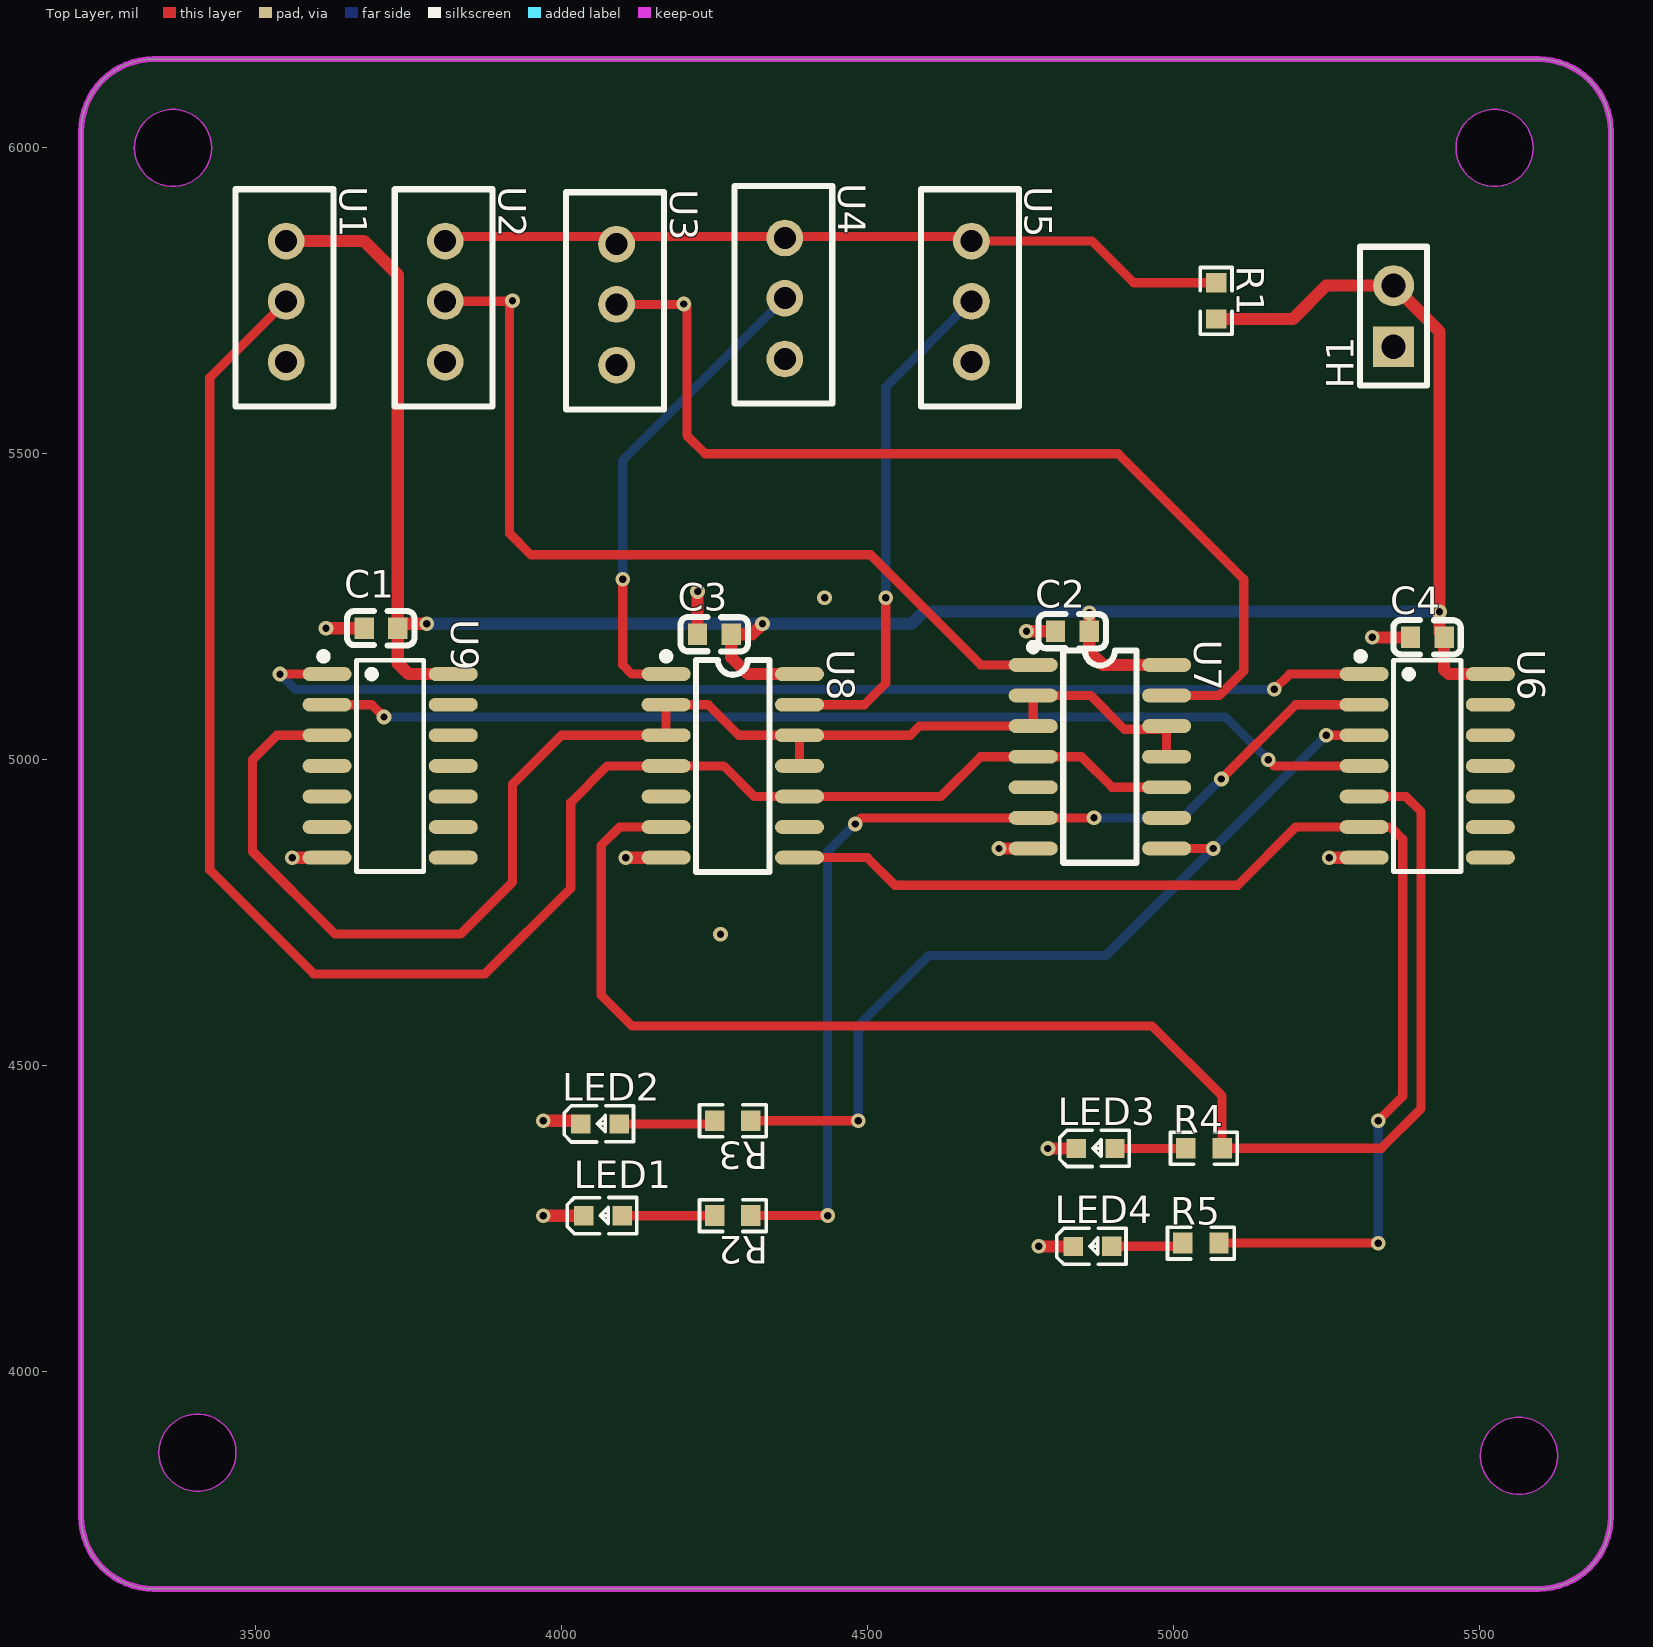
[diagram p0: Top Layer view]
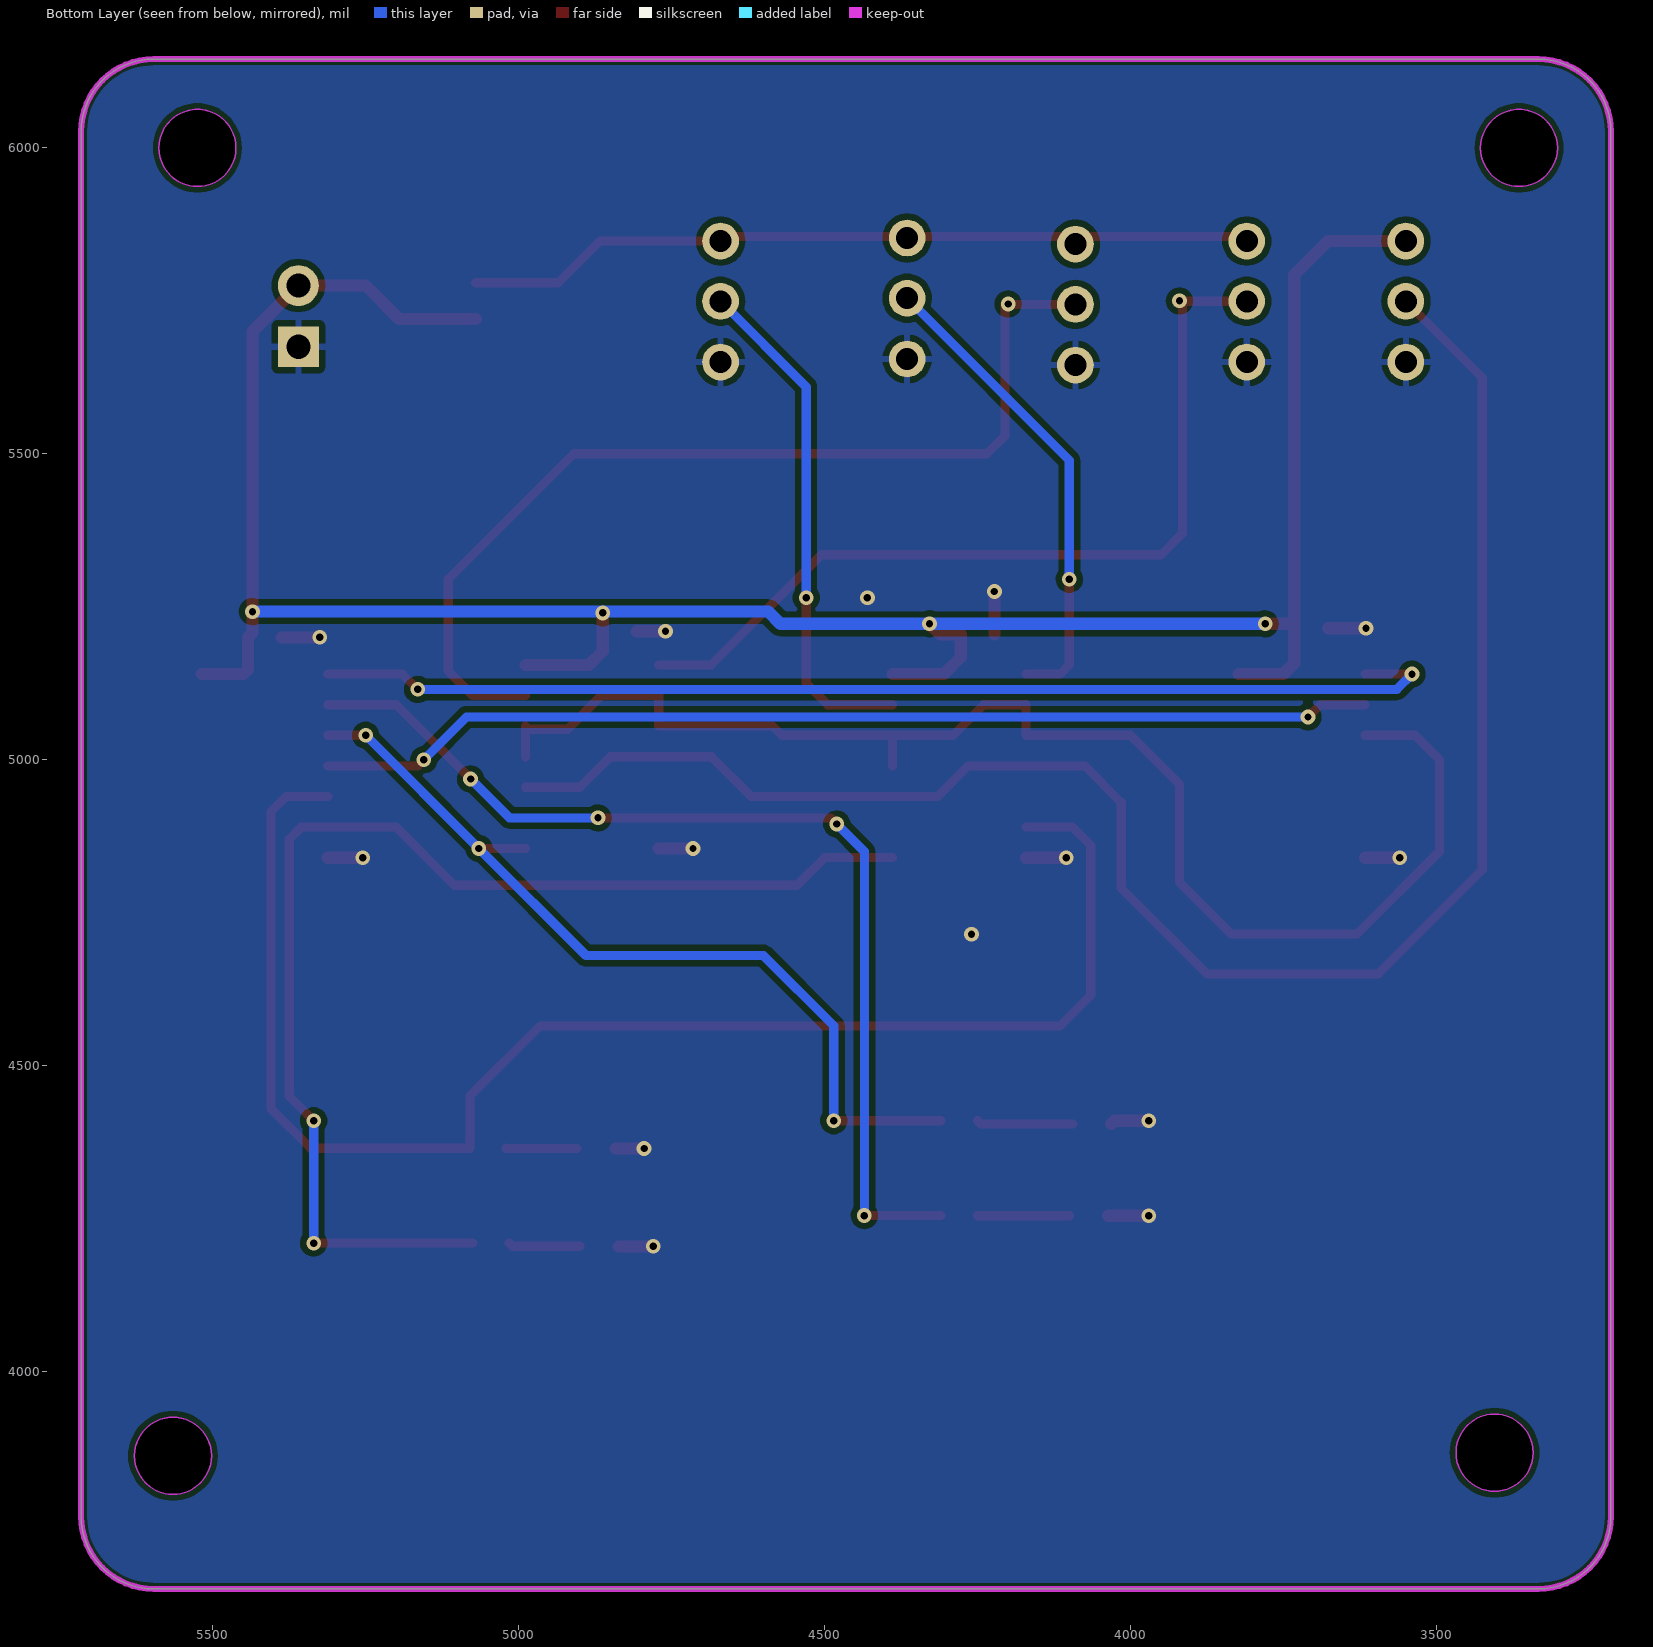
[diagram p1: Bottom Layer view, seen from below]
# Altium PCB MISC51255.pcbdoc
Units mil, origin at the board's own origin, x right, y up, seen from the top; angles counter-clockwise.
Board outline 2500 x 2500 mil, 2 copper layers (Top Layer, Bottom Layer), stack 62.206 mil thick; 23 components, 19 nets, 99 pads, 35 vias.

## Layer stack, top to bottom
Top Solder Mask Layer: solder mask 0.394, Dk 3.3
Top Layer: signal copper 1.379
Dielectric1: surface 59.449, FR4, Dk 4.5
Bottom Layer: signal copper 1.378
Bottom Solder Mask Layer: solder mask 0.394, Dk 3.3

## Board outline
3333.1,6145 ccw(c3333.1,6026.9) 3215,6026.9 3215,3763.1 ccw(c3333.1,3763.1) 3333.1,3645 5596.9,3645 ccw(c5596.9,3763.1) 5715,3763.1 5715,6026.9 ccw(c5596.9,6026.9) 5596.9,6145 3333.1,6145
cut-out: 3428,6000 cw(c3365,6000) 3302,6000 cw(c3365,6000)
cut-out: 5588,6000 cw(c5525,6000) 5462,6000 cw(c5525,6000)
cut-out: 3468,3867.44 cw(c3405,3867.44) 3342,3867.44 cw(c3405,3867.44)
cut-out: 5628,3862.44 cw(c5565,3862.44) 5502,3862.44 cw(c5565,3862.44)

## Design rules (kind name [scope] priority, off if disabled: settings)
BoardOutlineClearance copperThickness2oz_1 [All] p2 off: genericclearance=7.99 ignorepadtopadclearanceinfootprint=FALSE except(0: Arc-SplitContinuation Track-SplitContinuation SMDPad-SplitContinuation THPad-SplitContinuation Via-SplitContinuation Fill-SplitContinuation Region-SplitContinuation Poly-SplitContinuation Text-SplitContinuation Hole-SplitContinuation; 5.98: Arc-CutoutEdge SMDPad-CutoutEdge THPad-CutoutEdge Via-CutoutEdge Fill-CutoutEdge Region-CutoutEdge Text-CutoutEdge; 6.93: Hole-OutlineEdge Hole-CutoutEdge; 10: Poly-OutlineEdge Poly-CutoutEdge; 11.81: Arc-OutlineEdge Track-OutlineEdge SMDPad-OutlineEdge THPad-OutlineEdge Via-OutlineEdge Fill-OutlineEdge Region-OutlineEdge Text-OutlineEdge Track-CutoutEdge)
BoardOutlineClearance Plane_innerPlane_1 [All] p4 off: genericclearance=4.02 ignorepadtopadclearanceinfootprint=FALSE except(0: Arc-SplitContinuation Track-SplitContinuation SMDPad-SplitContinuation THPad-SplitContinuation Via-SplitContinuation Fill-SplitContinuation Region-SplitContinuation Poly-SplitContinuation Text-SplitContinuation Hole-SplitContinuation; 6: SMDPad-CutoutEdge THPad-CutoutEdge Via-CutoutEdge Fill-CutoutEdge Region-CutoutEdge Text-CutoutEdge; 6.93: Hole-OutlineEdge Hole-CutoutEdge; 10: Poly-OutlineEdge Poly-CutoutEdge; 11.8: Arc-OutlineEdge Track-OutlineEdge SMDPad-OutlineEdge THPad-OutlineEdge Via-OutlineEdge Fill-OutlineEdge Region-OutlineEdge Text-OutlineEdge; 11.81: Arc-CutoutEdge Track-CutoutEdge)
BoardOutlineClearance Copper_copperRegion_1 [All] p6 off: genericclearance=4.02 ignorepadtopadclearanceinfootprint=FALSE except(0: Arc-SplitContinuation Track-SplitContinuation SMDPad-SplitContinuation THPad-SplitContinuation Via-SplitContinuation Fill-SplitContinuation Region-SplitContinuation Poly-SplitContinuation Text-SplitContinuation Hole-SplitContinuation; 6: SMDPad-CutoutEdge THPad-CutoutEdge Via-CutoutEdge Fill-CutoutEdge Region-CutoutEdge Text-CutoutEdge; 6.93: Hole-OutlineEdge Hole-CutoutEdge; 10: Poly-OutlineEdge Poly-CutoutEdge; 11.8: Arc-OutlineEdge Track-OutlineEdge SMDPad-OutlineEdge THPad-OutlineEdge Via-OutlineEdge Fill-OutlineEdge Region-OutlineEdge Text-OutlineEdge; 11.81: Arc-CutoutEdge Track-CutoutEdge)
BoardOutlineClearance copperThickness1oz_1 [All] p8: genericclearance=4.02 ignorepadtopadclearanceinfootprint=FALSE except(0: Arc-SplitContinuation Track-SplitContinuation SMDPad-SplitContinuation THPad-SplitContinuation Via-SplitContinuation Fill-SplitContinuation Region-SplitContinuation Poly-SplitContinuation Text-SplitContinuation Hole-SplitContinuation; 6: SMDPad-CutoutEdge THPad-CutoutEdge Via-CutoutEdge Fill-CutoutEdge Region-CutoutEdge Text-CutoutEdge; 6.93: Hole-OutlineEdge Hole-CutoutEdge; 10: Poly-OutlineEdge Poly-CutoutEdge; 11.8: Arc-OutlineEdge Track-OutlineEdge SMDPad-OutlineEdge THPad-OutlineEdge Via-OutlineEdge Fill-OutlineEdge Region-OutlineEdge Text-OutlineEdge; 11.81: Arc-CutoutEdge Track-CutoutEdge)
Clearance copperThickness2oz [All] p1 off: gap=7.99 ignorepadtopadclearanceinfootprint=FALSE except(5.98: SMDPad-Track SMDPad-SMDPad THPad-Track SMDPad-THPad THPad-THPad Track-Via SMDPad-Via THPad-Via Via-Via Fill-Track Region-Track Fill-SMDPad Region-SMDPad Fill-THPad Region-THPad Fill-Via Region-Via Fill-Fill Fill-Region Region-Region Arc-Track Arc-SMDPad Arc-THPad Arc-Via Fill-Arc Region-Arc Arc-Arc Text-Track SMDPad-Text Text-THPad Text-Via Fill-Text Region-Text Arc-Text Text-Text; 6.93: Hole-Track Hole-SMDPad Hole-THPad Hole-Via Fill-Hole Region-Hole Hole-Arc Hole-Text; 10: Poly-Track Poly-SMDPad Poly-THPad Poly-Via Poly-Fill Poly-Region Poly-Poly Poly-Arc Poly-Text Poly-Hole)
Clearance Plane_innerPlane [All] p3 off: gap=4.02 ignorepadtopadclearanceinfootprint=FALSE except(5.98: SMDPad-Track SMDPad-SMDPad THPad-Track SMDPad-THPad THPad-THPad Track-Via SMDPad-Via THPad-Via Via-Via Fill-Track Region-Track Fill-SMDPad Region-SMDPad Fill-THPad Region-THPad Fill-Via Region-Via Fill-Fill Fill-Region Region-Region; 6: Arc-Track Arc-SMDPad Arc-THPad Arc-Via Fill-Arc Region-Arc Arc-Arc Text-Track SMDPad-Text Text-THPad Text-Via Fill-Text Region-Text Arc-Text Text-Text; 6.93: Hole-Track Hole-SMDPad Hole-THPad Hole-Via Fill-Hole Region-Hole Hole-Arc Hole-Text; 10: Poly-Track Poly-SMDPad Poly-THPad Poly-Via Poly-Fill Poly-Region Poly-Poly Poly-Arc Poly-Text Poly-Hole)
Clearance Copper_copperRegion [All] p5 off: gap=4.02 ignorepadtopadclearanceinfootprint=FALSE except(5.98: SMDPad-Track SMDPad-SMDPad THPad-Track SMDPad-THPad THPad-THPad Track-Via SMDPad-Via THPad-Via Via-Via Fill-Track Region-Track Fill-SMDPad Region-SMDPad Fill-THPad Region-THPad Fill-Via Region-Via Fill-Fill Fill-Region Region-Region; 6: Arc-Track Arc-SMDPad Arc-THPad Arc-Via Fill-Arc Region-Arc Arc-Arc Text-Track SMDPad-Text Text-THPad Text-Via Fill-Text Region-Text Arc-Text Text-Text; 6.93: Hole-Track Hole-SMDPad Hole-THPad Hole-Via Fill-Hole Region-Hole Hole-Arc Hole-Text; 10: Poly-Track Poly-SMDPad Poly-THPad Poly-Via Poly-Fill Poly-Region Poly-Poly Poly-Arc Poly-Text Poly-Hole)
Clearance copperThickness1oz [All] p7: gap=4.02 ignorepadtopadclearanceinfootprint=FALSE except(5.98: SMDPad-Track SMDPad-SMDPad THPad-Track SMDPad-THPad THPad-THPad Track-Via SMDPad-Via THPad-Via Via-Via Fill-Track Region-Track Fill-SMDPad Region-SMDPad Fill-THPad Region-THPad Fill-Via Region-Via Fill-Fill Fill-Region Region-Region; 6: Arc-Track Arc-SMDPad Arc-THPad Arc-Via Fill-Arc Region-Arc Arc-Arc Text-Track SMDPad-Text Text-THPad Text-Via Fill-Text Region-Text Arc-Text Text-Text; 6.93: Hole-Track Hole-SMDPad Hole-THPad Hole-Via Fill-Hole Region-Hole Hole-Arc Hole-Text; 10: Poly-Track Poly-SMDPad Poly-THPad Poly-Via Poly-Fill Poly-Region Poly-Poly Poly-Arc Poly-Text Poly-Hole)
DiffPairsRouting differentialPair [All] p1: maxlimit=6 minlimit=6 mostfreqgap=6 toplayer_minwidth=5 toplayer_prefwidth=10 toplayer_maxwidth=100 toplayer_mingap=6 toplayer_prefgap=6 toplayer_maxgap=6 bottomlayer_minwidth=5 bottomlayer_prefwidth=10 bottomlayer_maxwidth=100 bottomlayer_mingap=6 bottomlayer_prefgap=6 bottomlayer_maxgap=6 maxuncoupledlength=10
HoleToHoleClearance otherClearance [All] p1: gap=11.81 allowstackedmicrovias=TRUE
Length netLength [All] p1: minlimit=0 maxlimit=0
PasteMaskExpansion pasteMaskExpansion [All] p1: expansion=0
PlaneConnect innerPlane [All] p1: planeconnectstyle=Relief reliefexpansion=20 reliefentries=4 reliefconductorwidth=10 reliefairgap=10
PolygonConnect copperRegion [All] p1: connectstyle=Relief reliefconductorwidth=10 reliefentries=4 polygonreliefangle="90 Angle" airgapwidth=10 via.connectstyle=Relief via.reliefconductorwidth=10 via.reliefentries=4 via.polygonreliefangle="90 Angle" via.airgapwidth=10
RoutingVias viaSize [All] p1: holewidth=12.01 width=24.02 viastyle="Through Hole" minholewidth=11.81 minwidth=19.68 maxholewidth=248.03 maxwidth=393.7
SolderMaskExpansion solderMaskExpansion [IsVia] p1: expansion=-1000 istentingtop=TRUE
SolderMaskExpansion solderMaskExpansion [All] p2: expansion=2 istentingtop=FALSE
Width copperThickness2oz_2 [All] p1 off: maxlimit=100 minlimit=8 preferedwidth=10
Width pwr [(InNet('GND') OR InNet('VCC'))] p2: maxlimit=100 minlimit=5 preferedwidth=20
Width copperThickness1oz_2 [All] p3: maxlimit=100 minlimit=5 preferedwidth=15

## Components (designator, comment, footprint, x,y, rotation, side; value= is the part's Value field where it differs from the comment)
C1 "100nF" C0603 3705,5215 r0 top
C2 "100nF" C0603 4835,5210 r0 top
C3 "100nF" C0603 4250,5205 r0 top
C4 "100nF" C0603 5415,5200 r0 top
H1 "" HDR-TH_2P-P2.54-V-F 5360,5725 r90 top
LED1 "" LED_0603 4070,4255 r0 top
LED2 "" LED_0603 4065,4405 r0 top
LED3 "" LED_0603 4875,4365 r0 top
LED4 "" LED_0603 4870,4205 r0 top
R1 "0.1k" R0603 5070,5750 r270 top
R2 "10K" R0603 4280,4255 r180 top
R3 "10K" R0603 4280,4410 r180 top
R4 "10K" R0603 5050,4365 r180 top
R5 "10K" R0603 5045,4210 r180 top
U1 "" 单刀双掷 3680,5995 r270 top
U2 "" 单刀双掷 3940,5995 r270 top
U3 "" 单刀双掷 4220,5990 r270 top
U4 "" 单刀双掷 4495,6000 r270 top
U5 "" 单刀双掷 4800,5995 r270 top
U6 "SN74LS02DRE4" SOIC-14_L8.7-W3.9-P1.27-LS6.0-BL 5415,4990 r270 top
U7 "SN74LS113ADR" SOIC-14_L8.6-W3.9-P1.27-LS6.0-BL 4880,5005 r270 top
U8 "SN74LS113ADR" SOIC-14_L8.6-W3.9-P1.27-LS6.0-BL 4280,4990 r270 top
U9 "SN74LS08DTR(XBLW)" SOIC-14_L8.7-W3.9-P1.27-LS6.0-BL 3720,4990 r270 top

## Footprints (in the part's own frame and the unit in brackets; to place one, negate y for a bottom-side part, rotate by r counter-clockwise, add the part's x,y. Pads: shape width x height; smd on the part's side, far side on the other; paste and mask are expansions set on the pad)
C0603 [mm]
  rect 0.8x0.9 smd: 1(-0.7,0) 2(0.7,0)
  silkscreen extent -1.41,-0.71 1.39,0.72
HDR-TH_2P-P2.54-V-F [mm]
  rect 1.7x1.7 hole 1: 1(-1.27,0)
  round 1.7 hole 1: 2(1.27,0)
  silkscreen extent -2.88,-1.39 2.88,1.4
LED_0603 [mil]
  rect 31.5x31.5 smd paste+0 mask+2: 1(-33.5,-0.4) 2(29.5,-0.2)
  silkscreen extent -61,-30 53,30
R0603 [mil]
  rect 31.75x34.02 smd paste-3937.01 mask+2: 1(-29.66,0) 2(29.66,0)
  silkscreen extent -55,-26 55,26
SOIC-14_L8.6-W3.9-P1.27-LS6.0-BL [mil]
  oval 22.6x80.24 smd: 1(-150,-109.02) 2(-100,-109.02) 3(-50,-109.02) 4(0,-109.02) 5(50,-109.02) 6(100,-109.02) 7(150,-109.02) 8(150,109.02) 9(100,109.02) 10(50,109.02) 11(0,109.02) 12(-50,109.02) 13(-100,109.02) 14(-150,109.02)
  silkscreen extent -185,-115 173,60
SOIC-14_L8.7-W3.9-P1.27-LS6.0-BL [mil]
  oval 22.6x80.24 smd: 1(-150,-103.11) 2(-100,-103.11) 3(-50,-103.11) 4(0,-103.11) 5(50,-103.11) 6(100,-103.11) 7(150,-103.11) 8(150,103.11) 9(100,103.11) 10(50,103.11) 11(0,103.11) 12(-50,103.11) 13(-100,103.11) 14(-150,103.11)
  silkscreen extent -185,-115 172,55
单刀双掷 [mil]
  round 60 hole 36: 1(147.28,-130) 2(245.7,-130) 3(345,-130)
  silkscreen extent 63,-212 418,-52

## Via types
v1: diameter 24.02, hole 12, Top Layer to Bottom Layer, 35 vias

## Nets (pads, with @x,y where several pads share a name; then routed paths per layer and width w, separated by ;. In a path a pad name is that pad's centre, name@x,y a point inside that pad or via, vN(x,y) a via of type N, cw(c..) or ccw(c..) an arc to the next point about the centre after c; other vN are vias at no path point)
$1N6: R1.1 U2.1 U3.1 U4.1 U5.1 | length 1291.2
  Top Layer w15: U2.1 3817.28,5855 U5.1@4670,5855 ; U5.1 4867.28,5847.72 4935.34,5779.66 R1.1
$1N11: LED1.2 R2.2 | length 150.9
  Top Layer w15: LED1.2 4250.14,4254.8 R2.2
$1N12: LED2.2 R3.2 | length 158
  Top Layer w15: LED2.2 4245.14,4404.8 R3.2
$1N13: LED3.2 R4.2 | length 115.9
  Top Layer w15: LED3.2 5020.14,4364.8 R4.2
$1N14: LED4.2 R5.2 | length 118
  Top Layer w15: LED4.2 5010.14,4204.8 R5.2
$1N18: U2.2 U7.1 | length 1436.4
  Top Layer w15: U2.2 v1@3919.3,5749.3 ; v1(3920,5750) v1@3919.3,5749.3 ; U7.1 4685,5155 4505,5335 3950,5335 3915,5370 3915,5745 v1@3919.3,5749.3
$1N19: U3.2 U7.13 | length 1625.2
  Top Layer w15: U3.2 4199.3,5744.3 v1(4200,5745) ; v1@4205,5745 4205,5530 4235,5500 4910,5500 5115,5295 5115,5145 5075,5105 U7.13
$1N21: U4.2 U8.1 | length 786.3
  Top Layer w15: v1(4100,5295) 4100,5155 4115,5140 U8.1
  Bottom Layer w15: v1(4100,5295) 4100,5489.3 U4.2
$1N22: U5.2 U8.13 | length 837.8
  Top Layer w15: U8.13 4495,5090 4530,5125 v1(4530,5265)
  Bottom Layer w15: v1(4530,5265) 4530,5609.3 U5.2
$1N25: R2.1 U6.2 U7.6 | length 1696.6
  Top Layer w15: R2.1 v1(4435,4255) ; v1(4480,4895) 4490,4905 U7.6 v1(4870.25,4905) ; v1(5078.57,4968.57) 5200,5090 U6.2
  Bottom Layer w15: v1(4435,4255) 4435,4850 v1(4480,4895) ; v1(4870.25,4905) 5015,4905 v1(5078.57,4968.57)
$1N28: R5.1 U6.6 U8.8 | length 1989.2
  Top Layer w15: U8.8 4500,4840 4545,4795 5105,4795 5200,4890 U6.6 5355,4890 5375,4870 5375,4450 v1(5335,4410) ; R5.1 v1(5335,4210)
  Bottom Layer w15: v1(5335,4210) v1(5335,4410)
$1N35: U6.1 U9.1 | length 1869.5
  Top Layer w15: v1(3540,5140) U9.1 ; v1(5165,5115) 5190,5140 U6.1
  Bottom Layer w15: v1(3540,5140) 3565,5115 v1(5165,5115)
$1N36: U6.4 U9.2 | length 1736.4
  Top Layer w15: U9.2 3690,5090 v1(3710,5070) ; v1(5155,5000) 5165,4990 U6.4
  Bottom Layer w15: v1(3710,5070) 5085,5070 v1(5155,5000)
$1N44: R4.1 U6.5 U8.6 | length 2472.3
  Top Layer w15: U8.6 4095,4890 4065,4860 4065,4615 4115,4565 4965,4565 5079.66,4450.34 R4.1 5340,4365 5405,4430 5405,4915 5380,4940 U6.5
$1N47: U7.2 U7.3 U7.11 U7.12 U8.2 U8.3 U8.11 U8.12 U9.3 | length 2318.5
  Top Layer w15: U9.3 3535,5040 3495,5000 3495,4850 3630,4715 3835,4715 3920,4800 3920,4960 4000,5040 U8.3 U8.2 4240,5090 4290,5040 U8.12 ; U8.11 U8.12 ; U7.11 U7.12 4984.02,5050 4920,5050 4865,5105 U7.2 U7.3 4585,5055 4570,5040 U8.12
$1N50: U1.2 U7.4 U7.10 U8.4 U8.10 | length 2906.7
  Top Layer w15: U1.2 3425,5624.3 3425,4820 3595,4650 3875,4650 4015,4790 4015,4930 4075,4990 U8.4 4265,4990 4315,4940 U8.10 4620,4940 4685,5005 U7.4 4850,5005 4900,4955 U7.10
$1N52: R3.1 U6.3 U7.8 | length 1430
  Top Layer w15: R3.1 v1(4485,4410) ; U7.8 v1(5065,4855) ; v1(5250,5040) U6.3
  Bottom Layer w15: v1(4485,4410) 4485,4565 4600,4680 4890,4680 v1(5065,4855) v1(5250,5040)
GND: C1.1 C2.1 C3.1 C4.1 H1.1 LED1.1 LED2.1 LED3.1 LED4.1 U1.3 U2.3 U3.3 U4.3 U5.3 U6.7 U7.7 U8.7 U9.7 | length 711.5
  Top Layer w20: v1(3560,4840) U9.7 ; v1(3615,5215) C1.1 ; v1(3970,4254.6) LED1.1 ; v1(3970,4410) 4026.1,4410 LED2.1 ; v1(4105,4840) U8.7 ; C3.1 v1(4222.44,5275) ; v1(4715,4855) U7.7 ; v1(4760,5210) C2.1 ; v1(4780,4205) 4780.4,4204.6 LED4.1 ; v1(4795,4364.6) LED3.1 ; v1(5255,4840) U6.7 ; v1(5325,5200) C4.1
  other v1: 4260,4715 4430,5265
VCC: C1.2 C2.2 C3.2 C4.2 H1.2 R1.2 U1.1 U6.14 U7.14 U8.14 U9.14 | length 4121.6
  Top Layer w20: U1.1 3677.28,5847.72 3732.56,5792.44 C1.2 ; v1(3780,5222.11) 3739.67,5222.11 C1.2 ; U9.14 3750,5140 3732.56,5157.44 C1.2 ; v1(4328.48,5222.11) 4311.38,5205 C3.2 4277.56,5167.44 4305,5140 U8.14 ; v1(4862.56,5240) C2.2 4862.56,5177.44 4885,5155 U7.14 ; R1.2 5195.34,5720.34 5250,5775 H1.2 5435,5700 v1(5435,5242.11) 5435,5207.56 C4.2 5442.56,5147.44 5450,5140 U6.14
  Bottom Layer w20: v1(3780,5222.11) v1(4328.48,5222.11) 4572.11,5222.11 4592.11,5242.11 v1(5435,5242.11)
pads on no net: U6.8 U6.9 U6.10 U6.11 U6.12 U6.13 U7.5 U7.9 U8.5 U8.9 U9.4 U9.5 U9.6 U9.8 U9.9 U9.10 U9.11 U9.12 U9.13

## Polygon pours and split planes (outlines as drawn)
GND on Bottom Layer (solid, remove dead copper, pour order 0): 3000,6305 3000,3230 6280,3230 6280,6305
GND on Bottom Layer (solid, remove dead copper, pour order 0): 3165,6070 3165,3000 6415,3000 6415,6070

## Keep-outs
Board Outline Layer:
  region: 3428,6000 cw(c3365,6000) 3302,6000 cw(c3365,6000)
  circle w0.1: c3365,6000 r63
  region: 3428,6000 3427.6,5992.95 3426.42,5985.98 3424.46,5979.19 3421.76,5972.67 3418.34,5966.48 3414.26,5960.72 3409.55,5955.45 3404.28,5950.74 3398.52,5946.66 3392.33,5943.24 3385.81,5940.54 3379.02,5938.58 3372.05,5937.4 3365,5937 3357.95,5937.4 3350.98,5938.58 3344.19,5940.54 3337.67,5943.24 3331.48,5946.66 3325.72,5950.74 3320.45,5955.45 3315.74,5960.72 3311.66,5966.48 3308.24,5972.67 3305.54,5979.19 3303.58,5985.98 3302.4,5992.95 3302,6000 3302.4,6007.05 3303.58,6014.02 3305.54,6020.81 3308.24,6027.33 3311.66,6033.52 3315.74,6039.28 3320.45,6044.55 3325.72,6049.26 3331.48,6053.34 3337.67,6056.76 3344.19,6059.46 3350.98,6061.42 3357.95,6062.6 3365,6063 3372.05,6062.6 3379.02,6061.42 3385.81,6059.46 3392.33,6056.76 3398.52,6053.34 3404.28,6049.26 3409.55,6044.55 3414.26,6039.28 3418.34,6033.52 3421.76,6027.33 3424.46,6020.81 3426.42,6014.02 3427.6,6007.05
  region: 5588,6000 cw(c5525,6000) 5462,6000 cw(c5525,6000)
  circle w0.1: c5525,6000 r63
  region: 5588,6000 5587.6,5992.95 5586.42,5985.98 5584.46,5979.19 5581.76,5972.67 5578.34,5966.48 5574.26,5960.72 5569.55,5955.45 5564.28,5950.74 5558.52,5946.66 5552.33,5943.24 5545.81,5940.54 5539.02,5938.58 5532.05,5937.4 5525,5937 5517.95,5937.4 5510.98,5938.58 5504.19,5940.54 5497.67,5943.24 5491.48,5946.66 5485.72,5950.74 5480.45,5955.45 5475.74,5960.72 5471.66,5966.48 5468.24,5972.67 5465.54,5979.19 5463.58,5985.98 5462.4,5992.95 5462,6000 5462.4,6007.05 5463.58,6014.02 5465.54,6020.81 5468.24,6027.33 5471.66,6033.52 5475.74,6039.28 5480.45,6044.55 5485.72,6049.26 5491.48,6053.34 5497.67,6056.76 5504.19,6059.46 5510.98,6061.42 5517.95,6062.6 5525,6063 5532.05,6062.6 5539.02,6061.42 5545.81,6059.46 5552.33,6056.76 5558.52,6053.34 5564.28,6049.26 5569.55,6044.55 5574.26,6039.28 5578.34,6033.52 5581.76,6027.33 5584.46,6020.81 5586.42,6014.02 5587.6,6007.05
  region: 3468,3867.44 cw(c3405,3867.44) 3342,3867.44 cw(c3405,3867.44)
  circle w0.1: c3405,3867.44 r63
  region: 3468,3867.44 3467.6,3860.39 3466.42,3853.42 3464.46,3846.63 3461.76,3840.11 3458.34,3833.92 3454.26,3828.16 3449.55,3822.89 3444.28,3818.19 3438.52,3814.1 3432.33,3810.68 3425.81,3807.98 3419.02,3806.02 3412.05,3804.84 3405,3804.44 3397.95,3804.84 3390.98,3806.02 3384.19,3807.98 3377.67,3810.68 3371.48,3814.1 3365.72,3818.19 3360.45,3822.89 3355.74,3828.16 3351.66,3833.92 3348.24,3840.11 3345.54,3846.63 3343.58,3853.42 3342.4,3860.39 3342,3867.44 3342.4,3874.5 3343.58,3881.46 3345.54,3888.25 3348.24,3894.78 3351.66,3900.96 3355.74,3906.72 3360.45,3911.99 3365.72,3916.7 3371.48,3920.79 3377.67,3924.2 3384.19,3926.91 3390.98,3928.86 3397.95,3930.05 3405,3930.44 3412.05,3930.05 3419.02,3928.86 3425.81,3926.91 3432.33,3924.2 3438.52,3920.79 3444.28,3916.7 3449.55,3911.99 3454.26,3906.72 3458.34,3900.96 3461.76,3894.78 3464.46,3888.25 3466.42,3881.46 3467.6,3874.5
  region: 5628,3862.44 cw(c5565,3862.44) 5502,3862.44 cw(c5565,3862.44)
  circle w0.1: c5565,3862.44 r63
  region: 5628,3862.44 5627.6,3855.39 5626.42,3848.42 5624.46,3841.63 5621.76,3835.11 5618.34,3828.92 5614.26,3823.16 5609.55,3817.89 5604.28,3813.19 5598.52,3809.1 5592.33,3805.68 5585.81,3802.98 5579.02,3801.02 5572.05,3799.84 5565,3799.44 5557.95,3799.84 5550.98,3801.02 5544.19,3802.98 5537.67,3805.68 5531.48,3809.1 5525.72,3813.19 5520.45,3817.89 5515.74,3823.16 5511.66,3828.92 5508.24,3835.11 5505.54,3841.63 5503.58,3848.42 5502.4,3855.39 5502,3862.44 5502.4,3869.5 5503.58,3876.46 5505.54,3883.25 5508.24,3889.78 5511.66,3895.96 5515.74,3901.72 5520.45,3906.99 5525.72,3911.7 5531.48,3915.79 5537.67,3919.2 5544.19,3921.91 5550.98,3923.86 5557.95,3925.05 5565,3925.44 5572.05,3925.05 5579.02,3923.86 5585.81,3921.91 5592.33,3919.2 5598.52,3915.79 5604.28,3911.7 5609.55,3906.99 5614.26,3901.72 5618.34,3895.96 5621.76,3889.78 5624.46,3883.25 5626.42,3876.46 5627.6,3869.5
  lines w10: 3215,3763.1 3215,6026.9 cw(c3333.1,6026.9) 3333.1,6145 5596.9,6145 cw(c5596.9,6026.9) 5715,6026.9 5715,3763.1 cw(c5596.9,3763.1) 5596.9,3645 3333.1,3645 cw(c3333.1,3763.1) 3215,3763.1

## Silkscreen, mask and mechanical layers (free items; w line width, h text height)
Mechanical Layer:
  circle w0.1: c3365,6000 r63
  circle w0.1: c5525,6000 r63
  circle w0.1: c3405,3867.44 r63
  circle w0.1: c5565,3862.44 r63